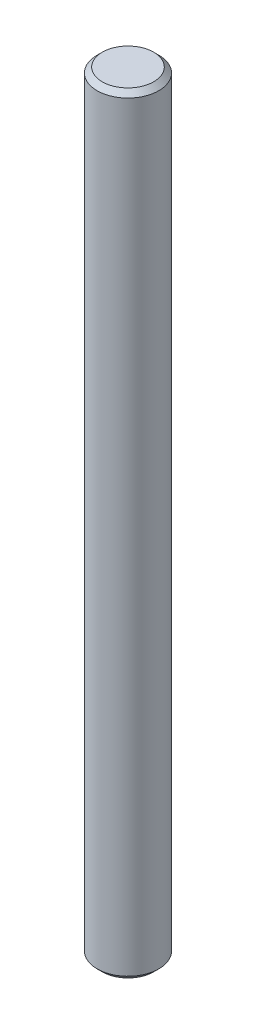
from build123d import *

# Parameters (mm, degrees)
SKETCH1_R           = 0.6
BOSS_EXTRUDE1_DEPTH = 15
CHAMFER1_SIZE       = 0.1


with BuildPart() as part:
    # Sketch1 → Boss-Extrude1 (new body)
    with BuildSketch(Plane(origin=(0, 0, 0), x_dir=(1, 0, 0), z_dir=(0, 1, 0))):
        with Locations(Location((0, 0, 0), (0, 0, 270))):
            Circle(SKETCH1_R)
    extrude(amount=BOSS_EXTRUDE1_DEPTH)

    # Chamfer1
    chamfer1_edges = [part.edges().sort_by_distance(p)[0] for p in [
        (0, 0, -0.6),
        (0, 15, -0.6),
    ]]
    chamfer(chamfer1_edges, length=CHAMFER1_SIZE)


solid = part.part
